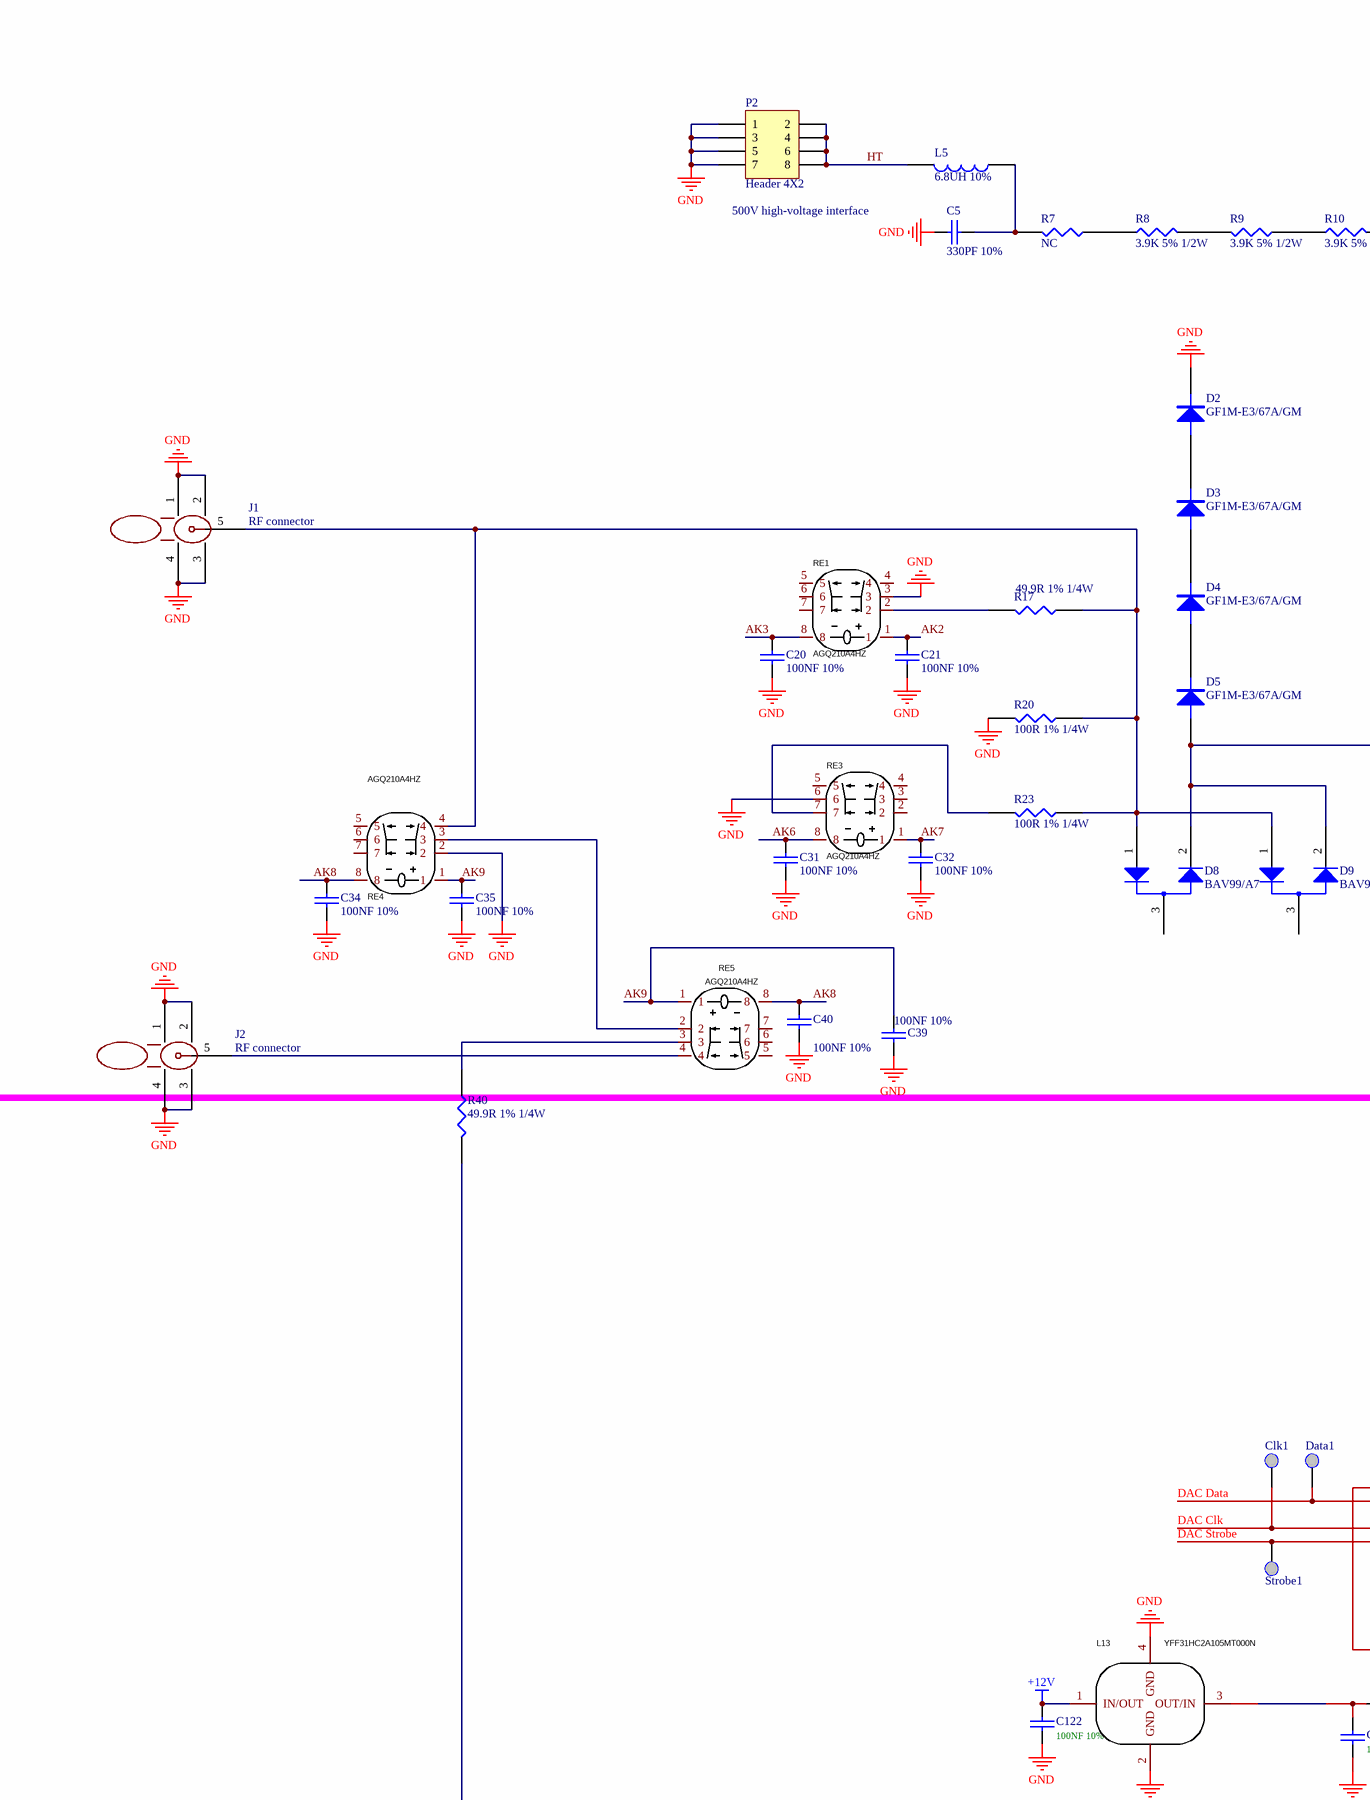
[diagram p0: PCBE109560.SchDoc, top left]
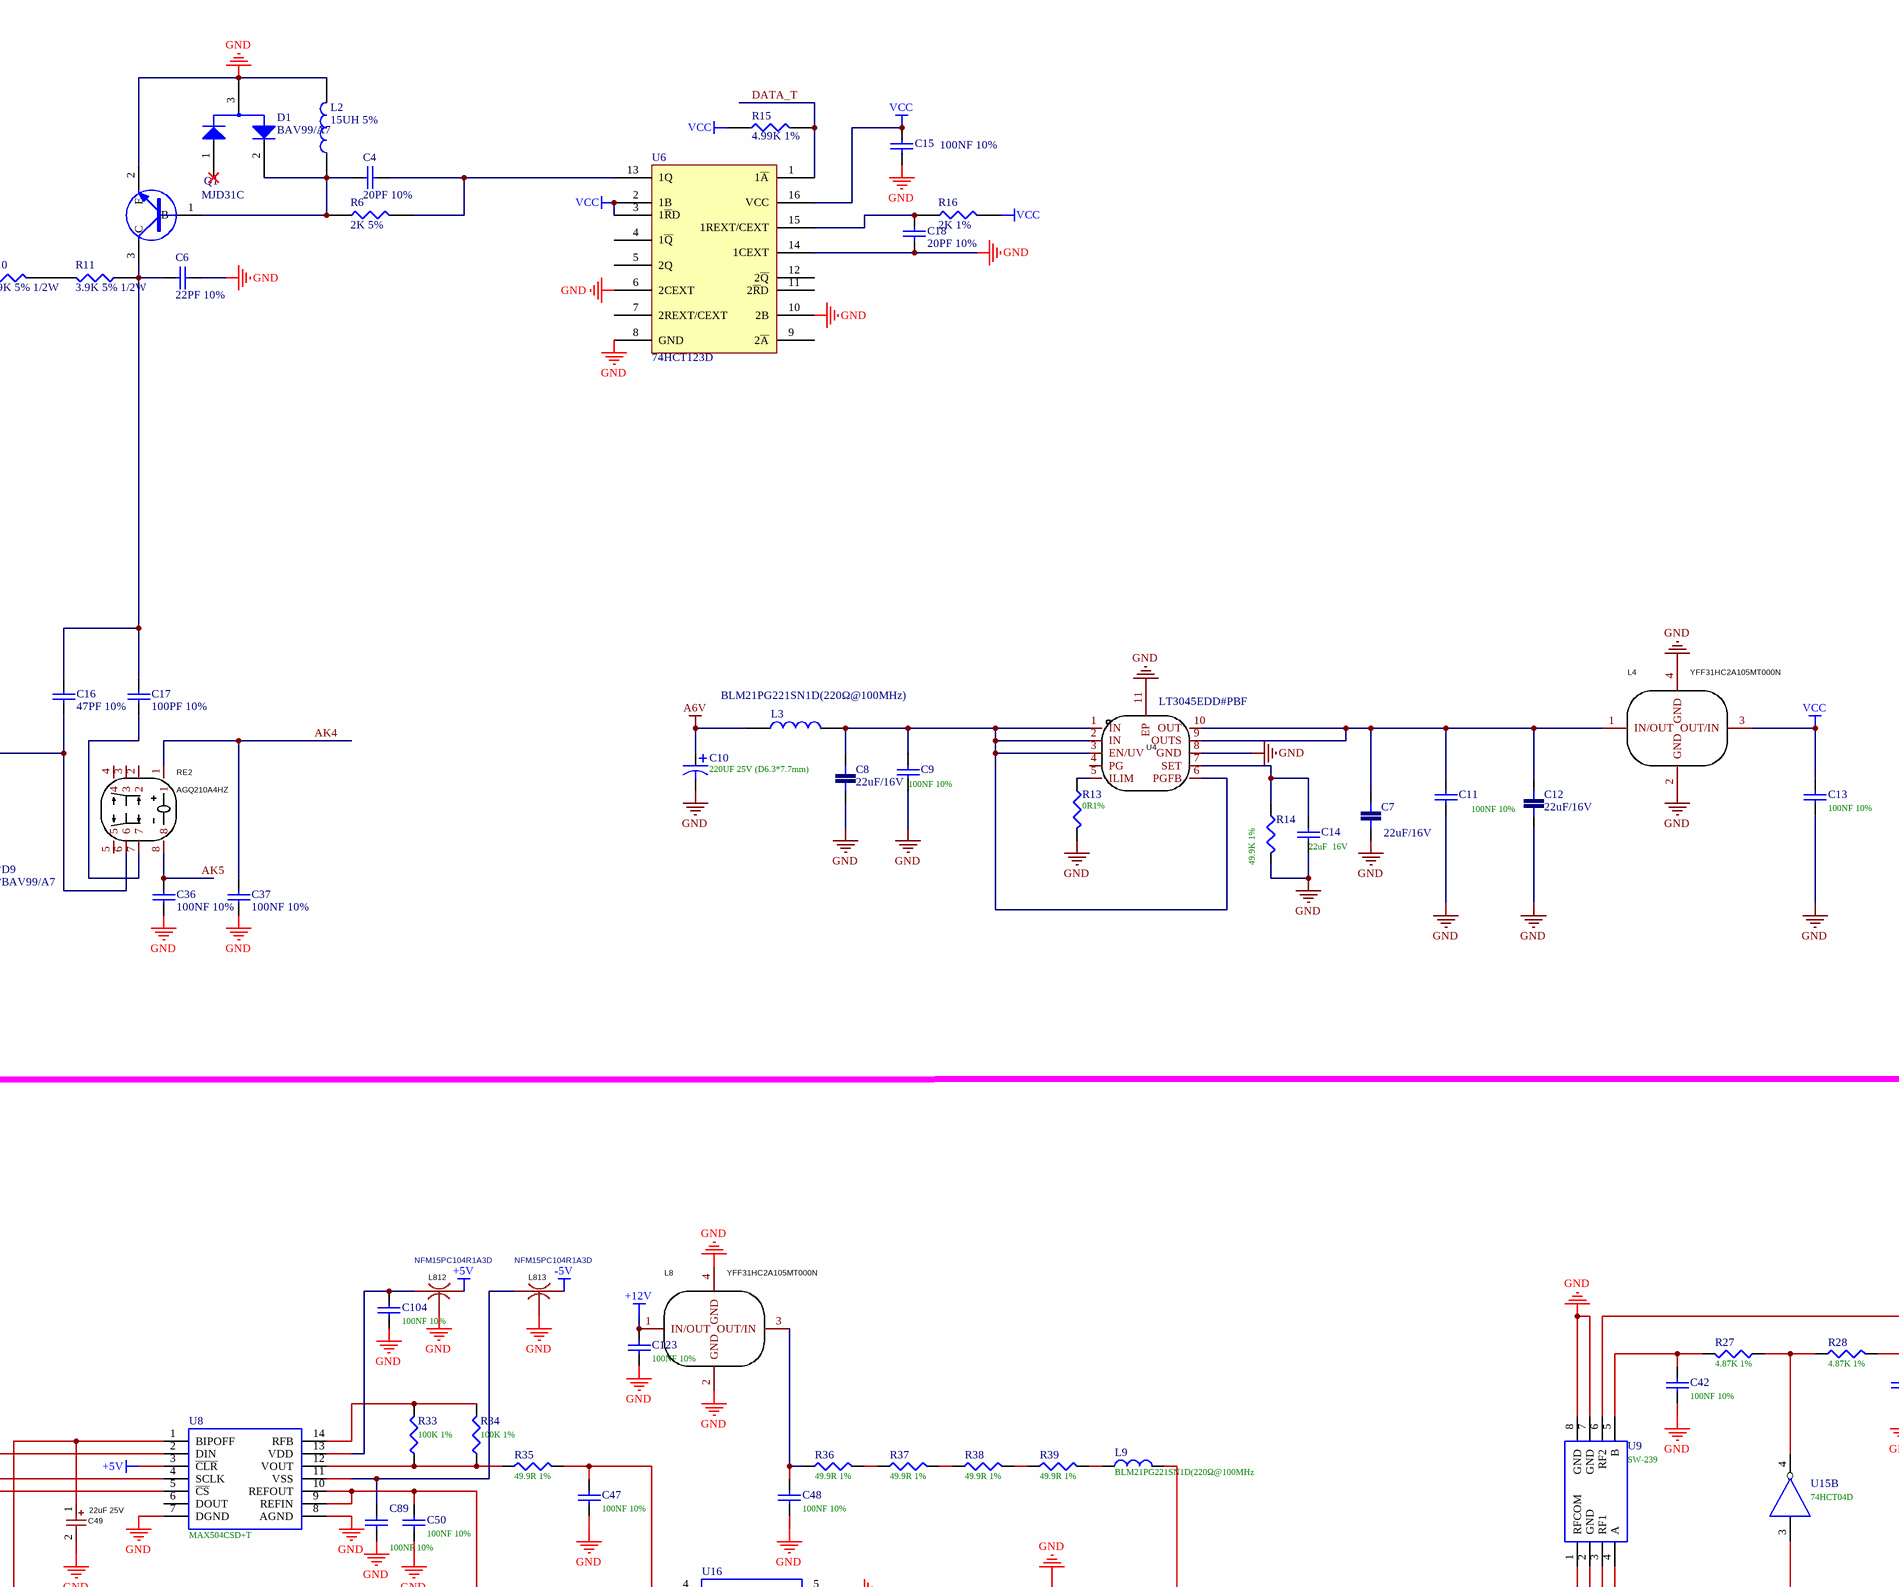
[diagram p1: PCBE109560.SchDoc, top middle]
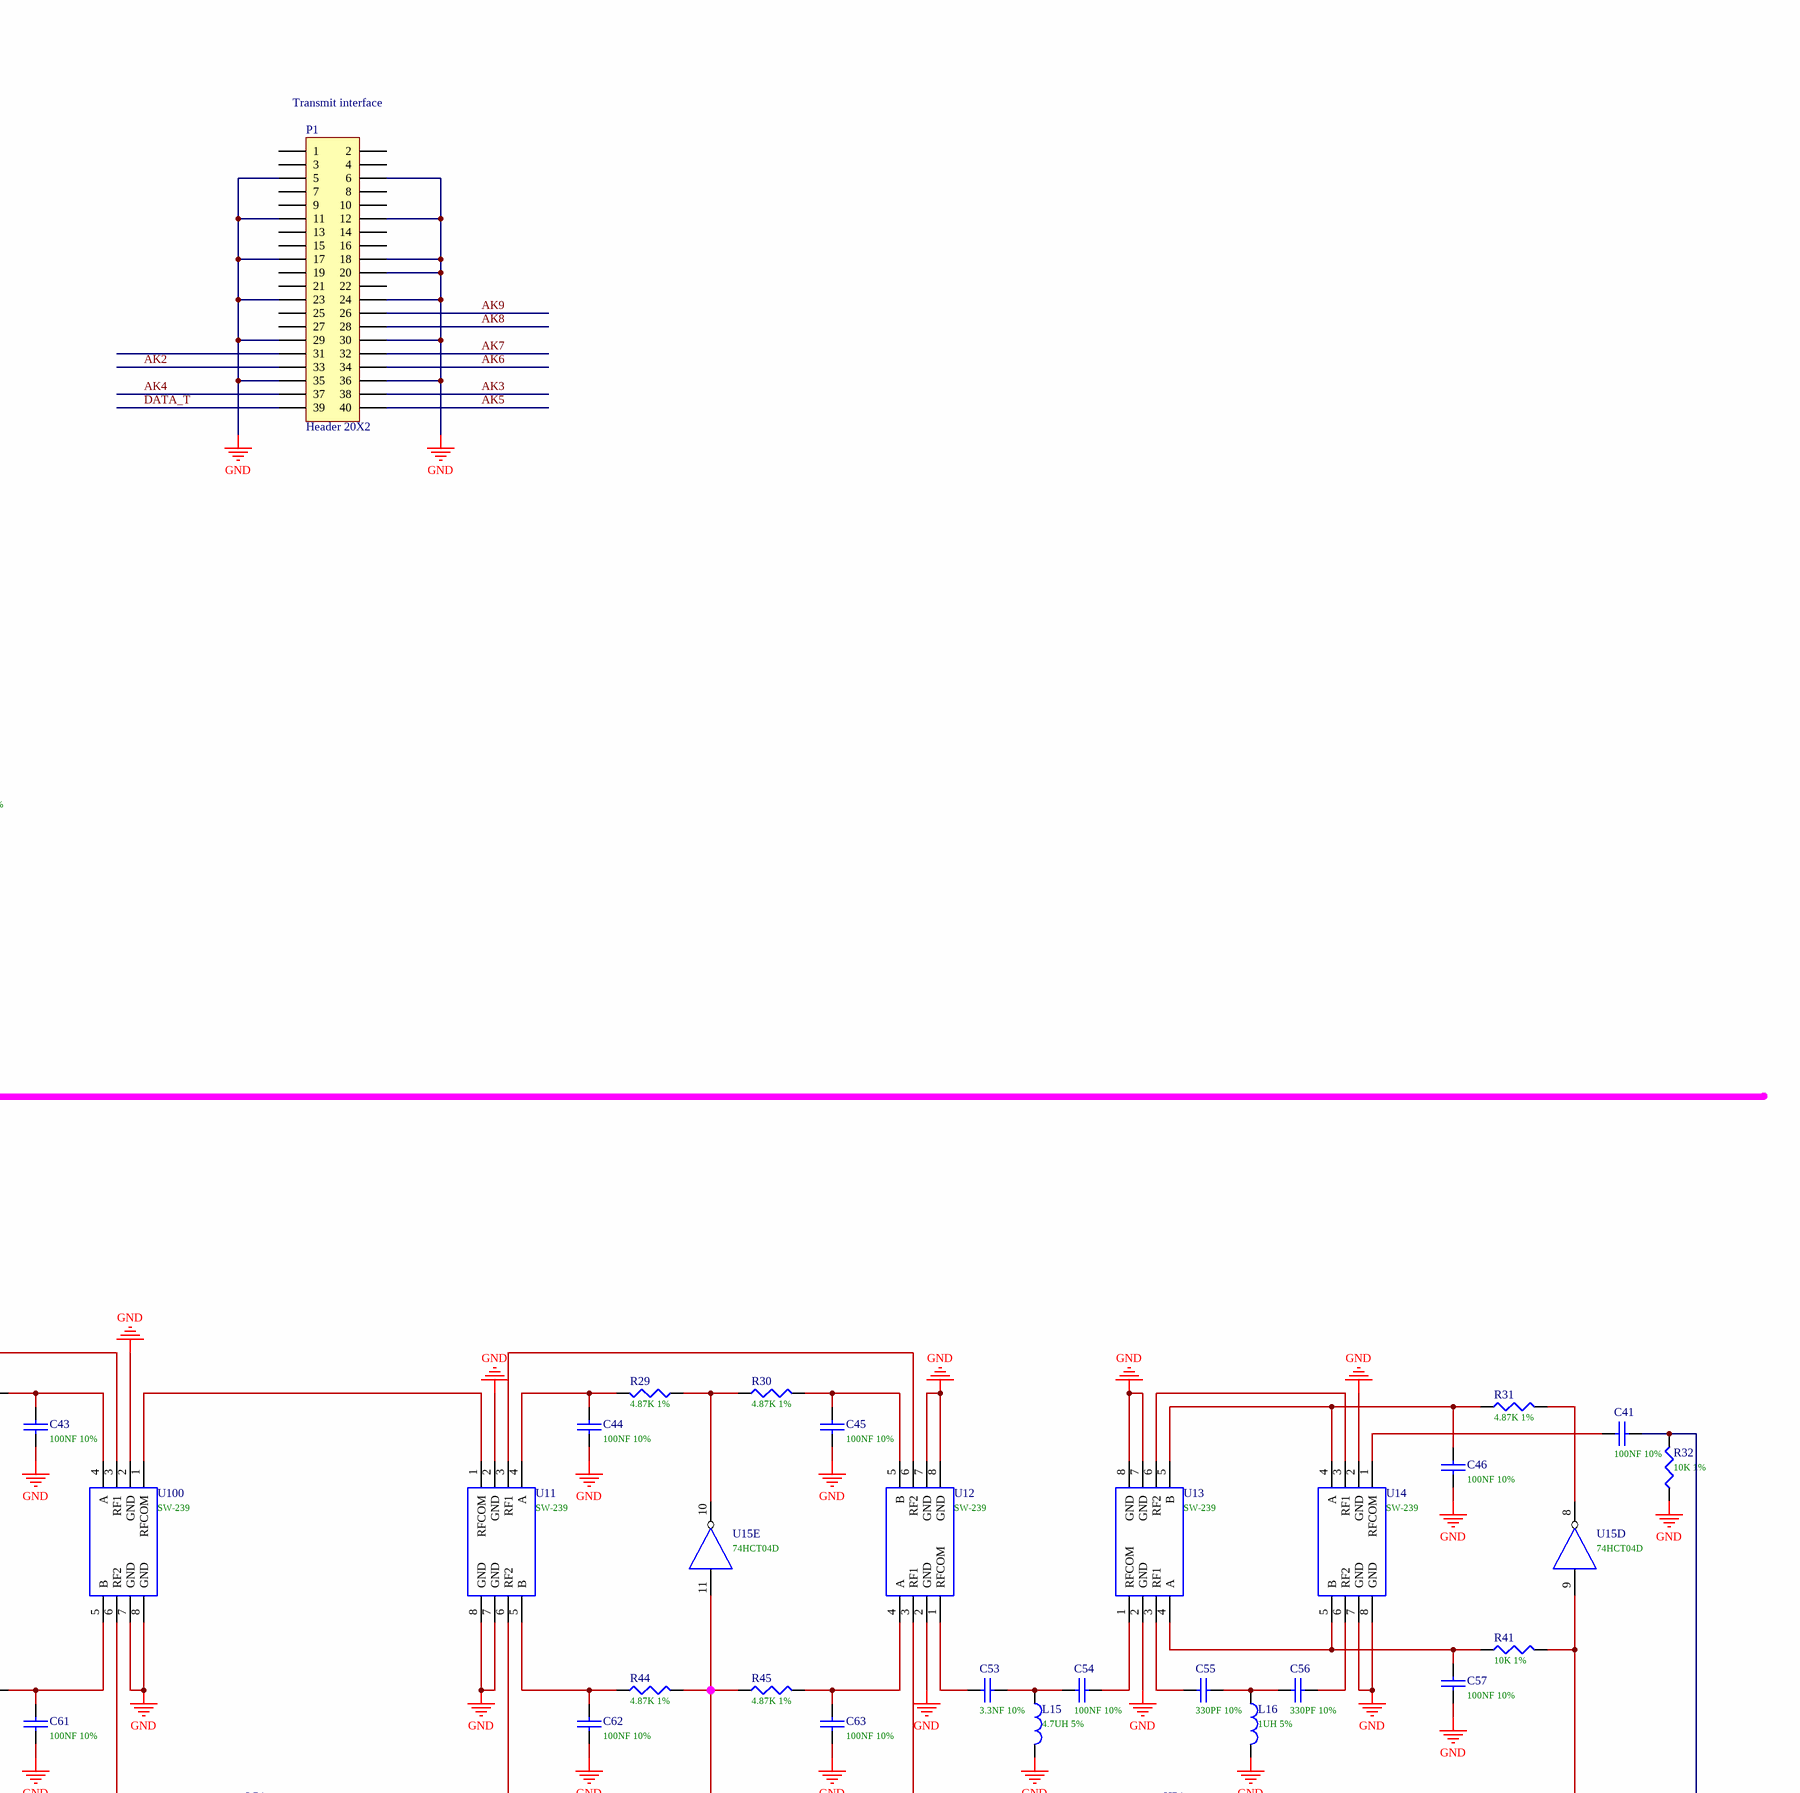
[diagram p2: PCBE109560.SchDoc, top right]
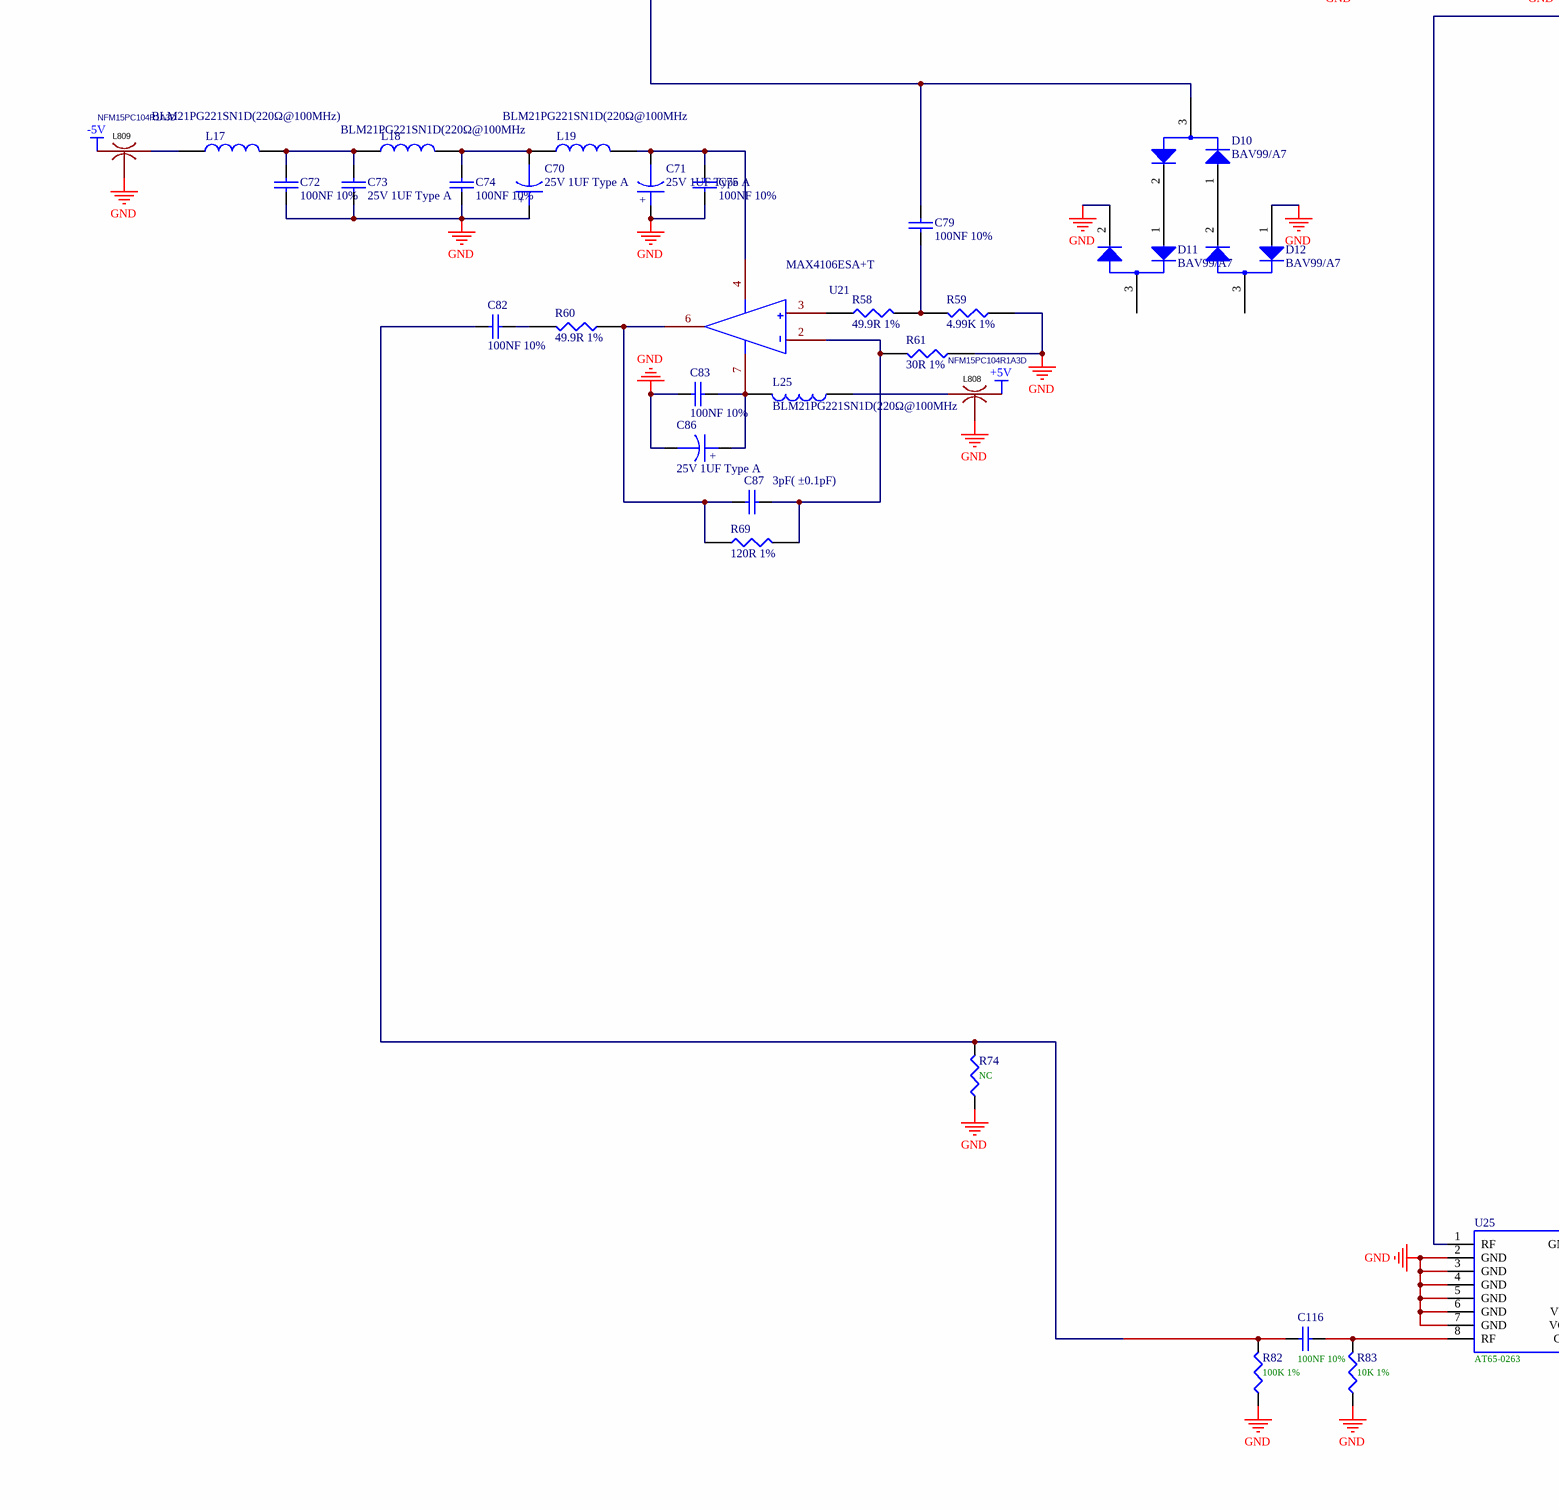
[diagram p3: PCBE109560.SchDoc, bottom left]
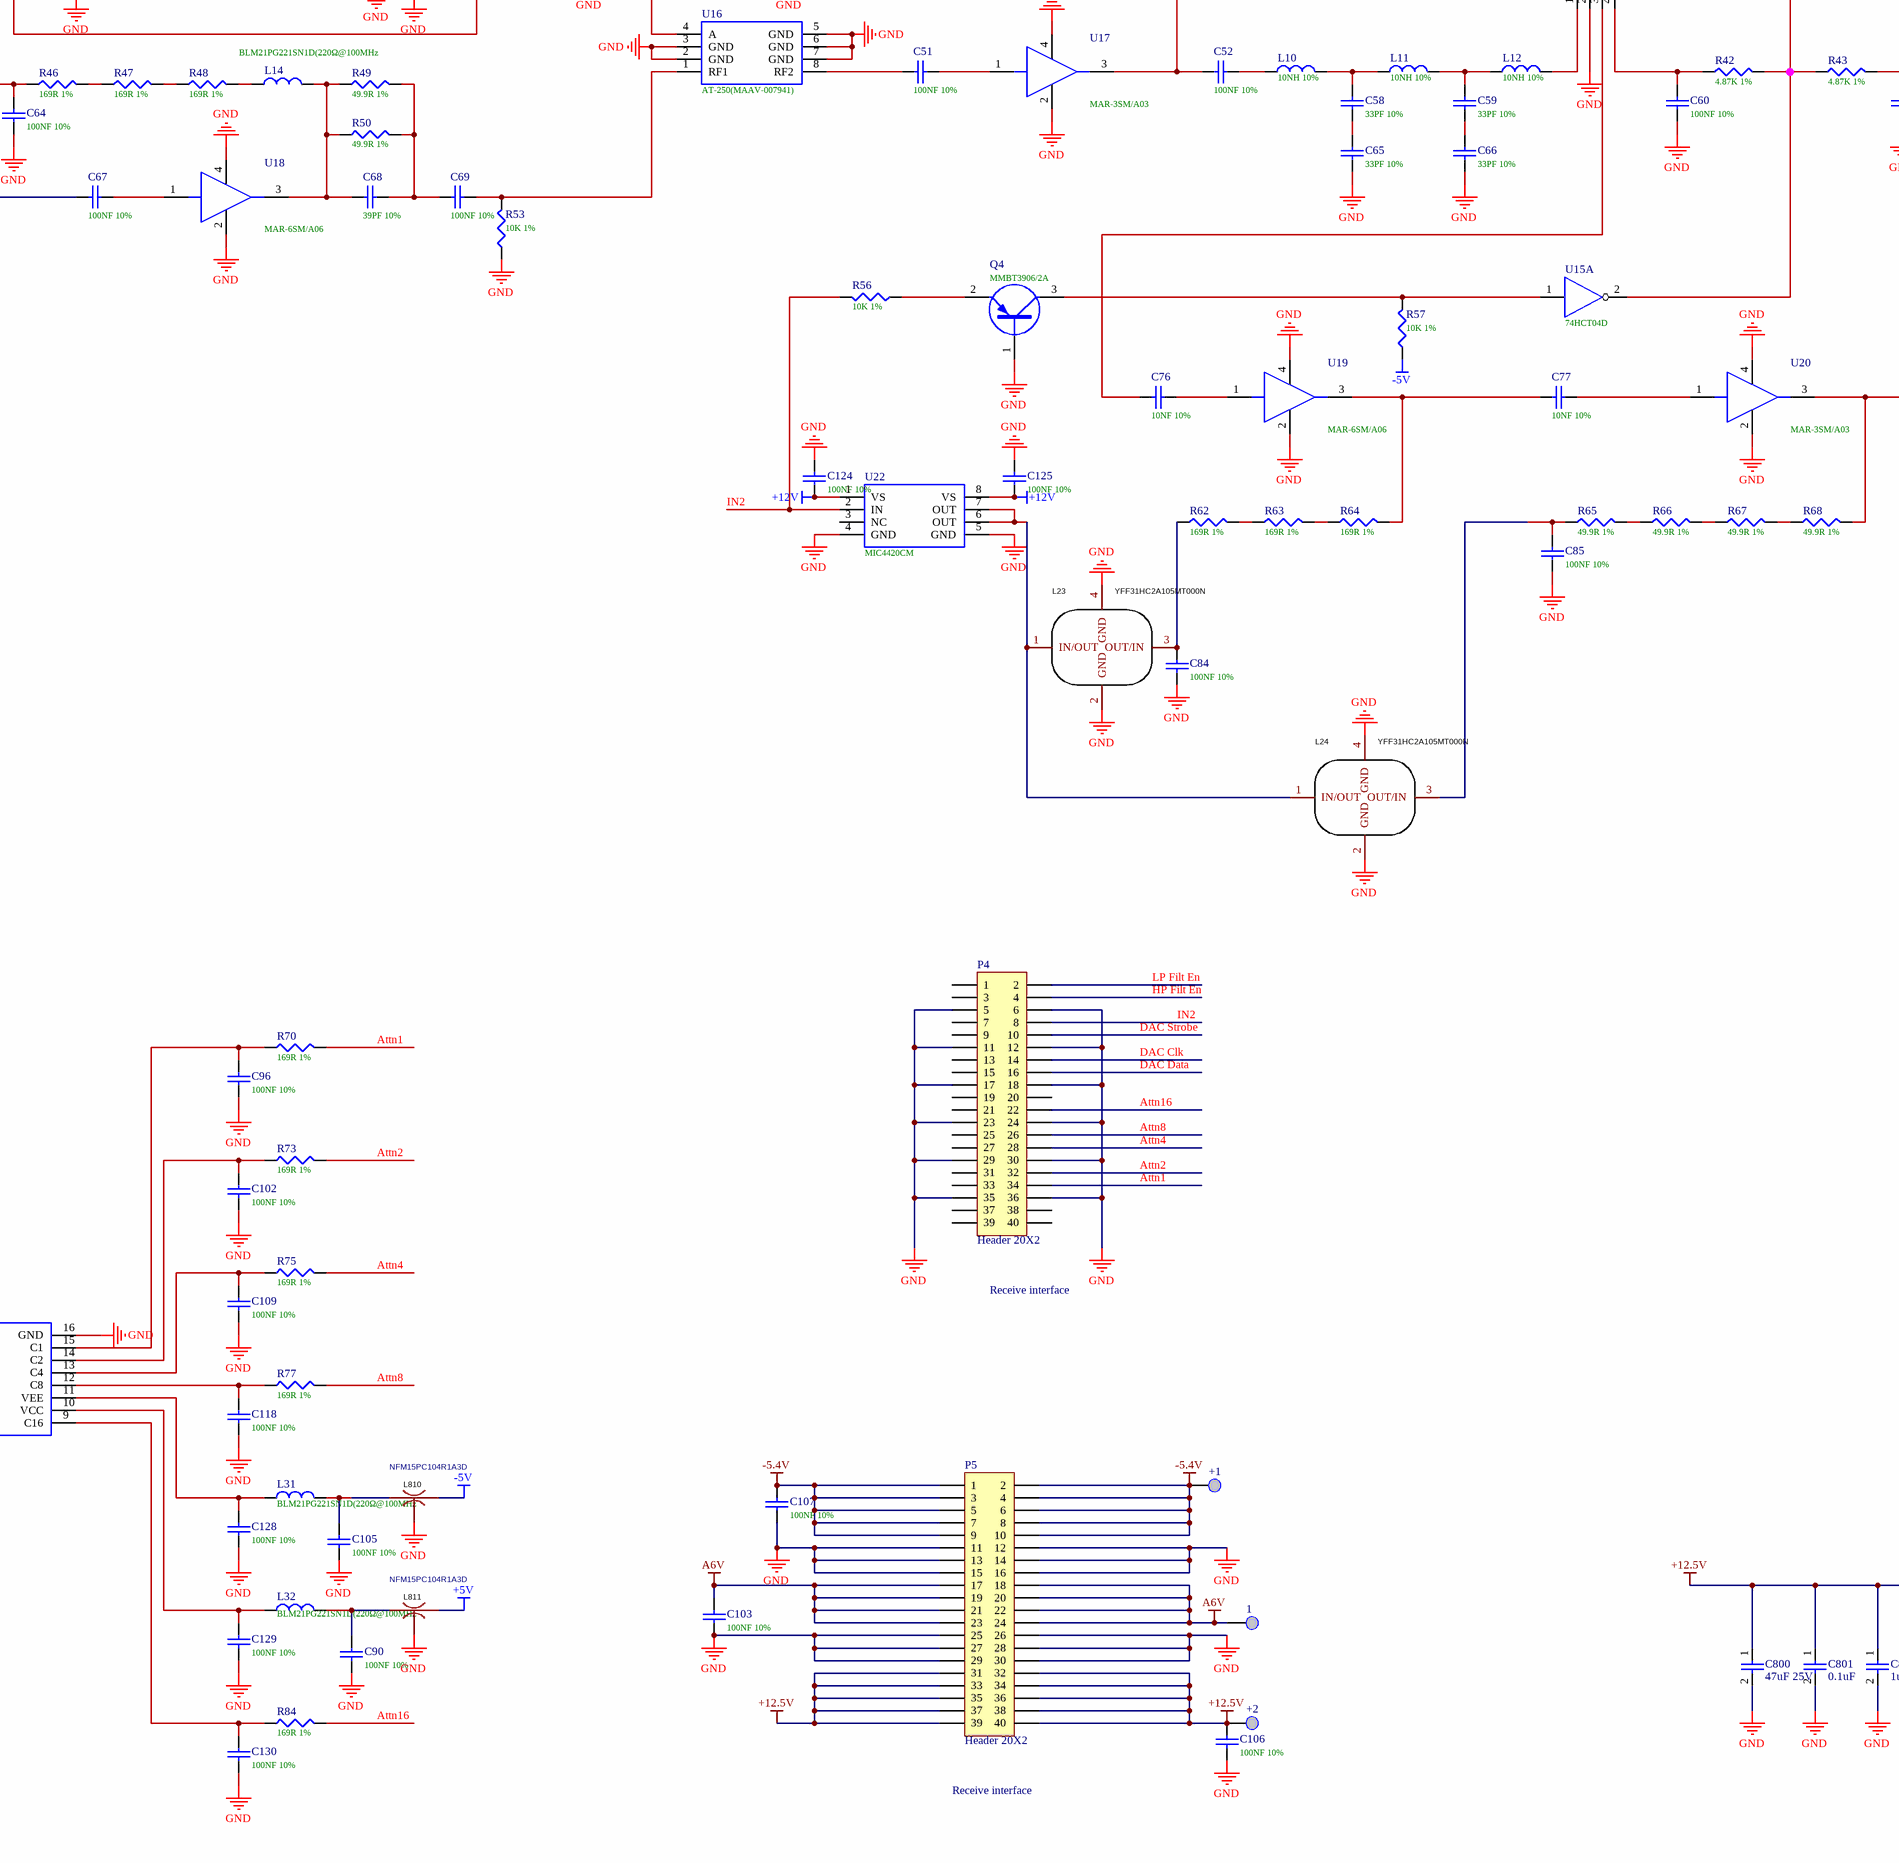
[diagram p4: PCBE109560.SchDoc, bottom middle]
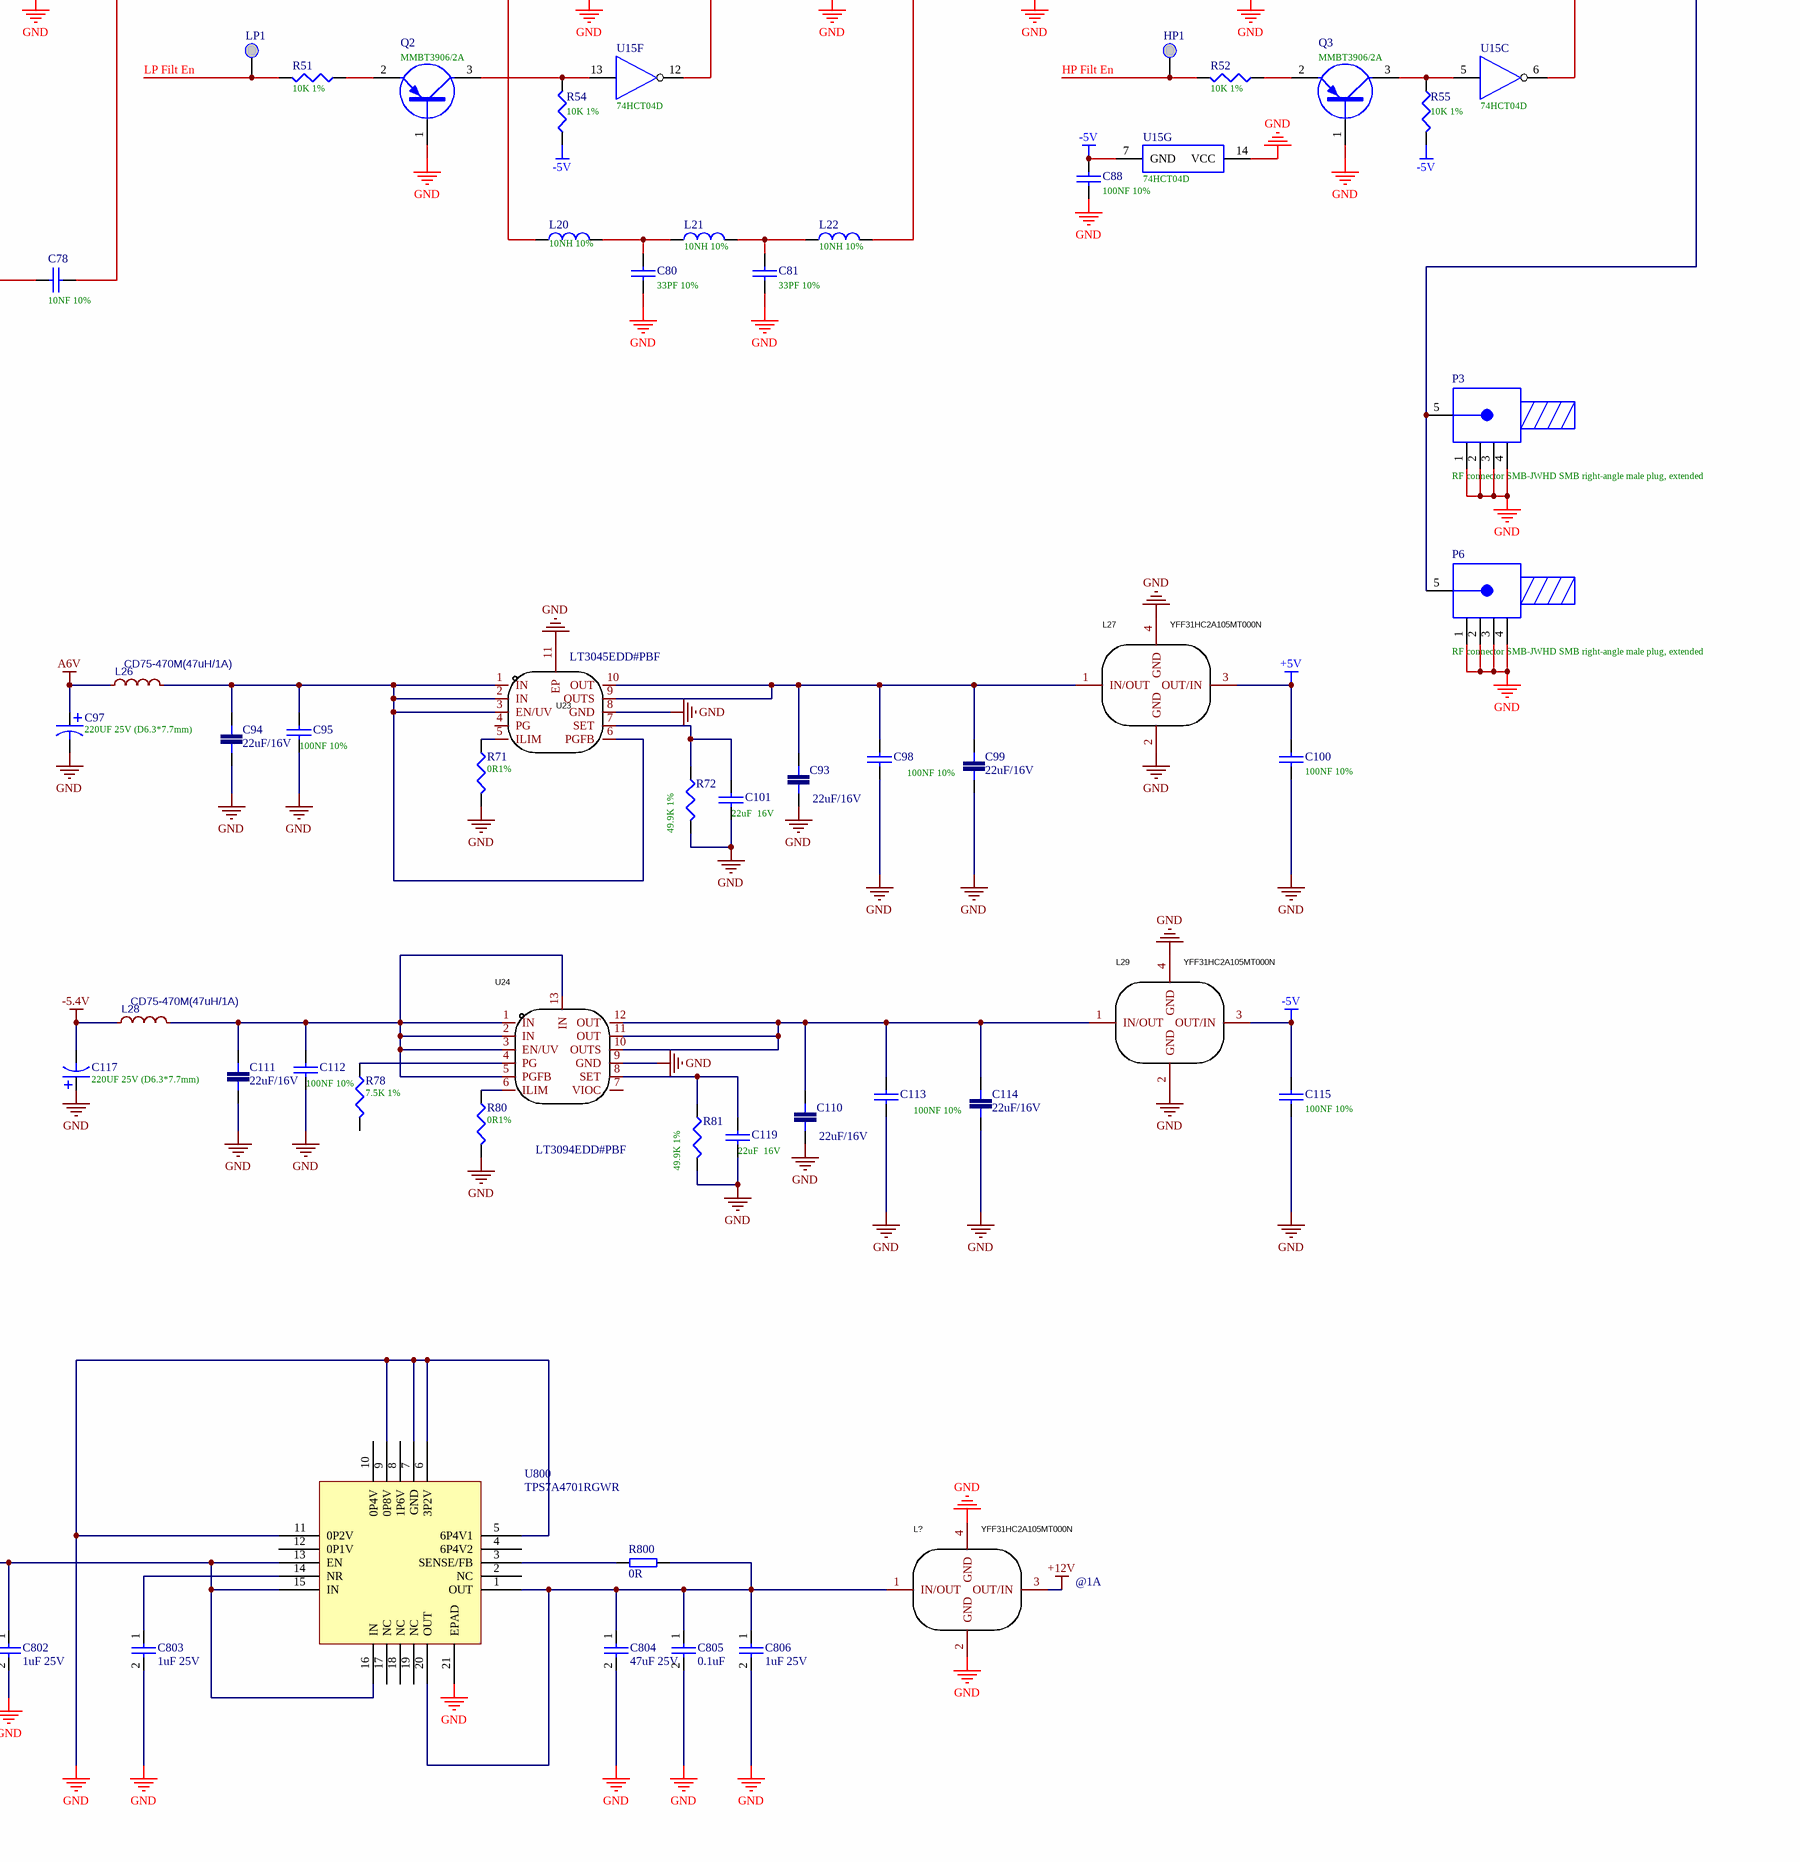
[diagram p5: PCBE109560.SchDoc, bottom right]
# Altium schematic sheet PCBE109560.SchDoc (part 1 of 2)
size E; SheetNumber: 0; SheetTotal: 0